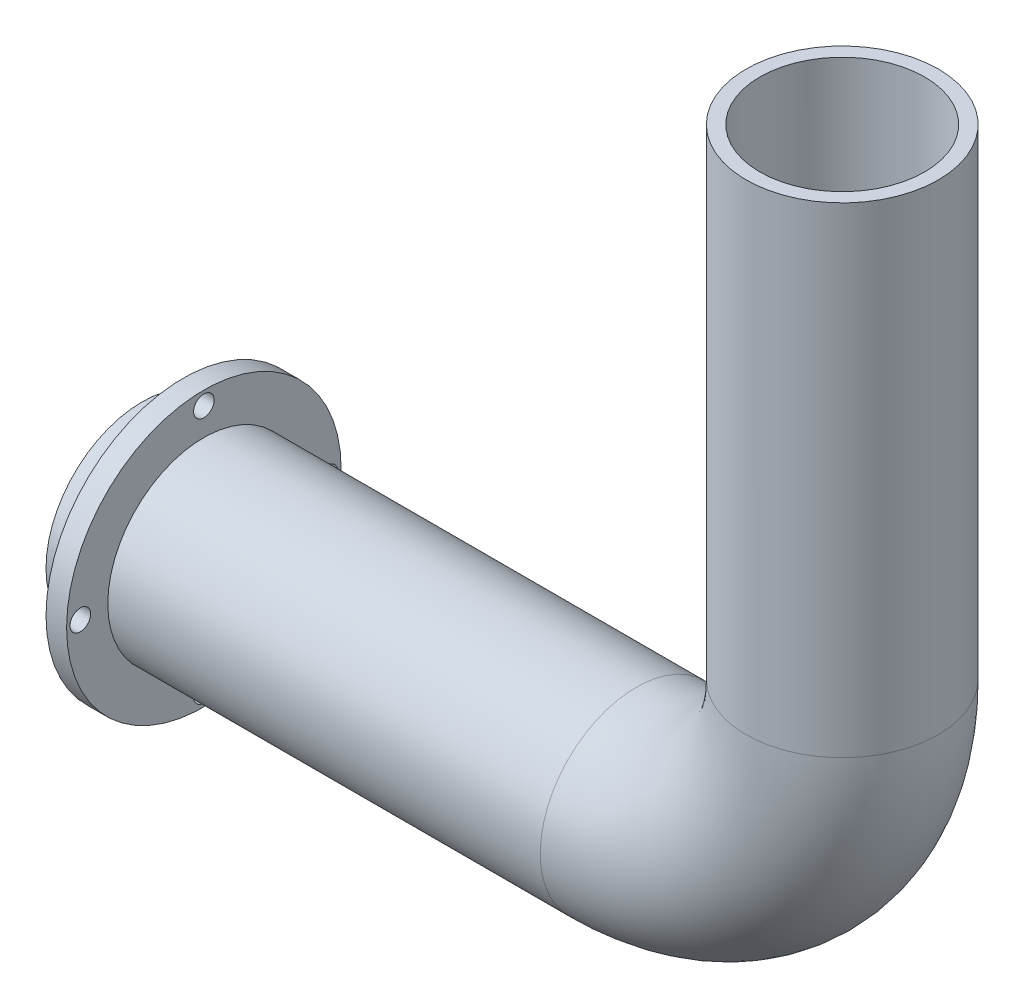
SolidWorks part; units mm, degrees
ref_plane "Front Plane" through (0, 0, 0) normal (0, 0, 1) x (1, 0, 0)
ref_plane "Top Plane" through (0, 0, 0) normal (0, 1, 0) x (1, 0, 0)
ref_plane "Right Plane" through (0, 0, 0) normal (1, 0, 0) x (0, 0, -1)
sketch "Sketch1" plane through (0, 0, 0) normal (0, 0, 1) x (1, 0, 0)
  line L0 (0, 0) -> (0, -70)
  line L1 (-30, -100) -> (-102, -100)
  arc A0 (0, -70) -> (-30, -100) centre (-30, -70) cw
  point P6 (0, -100)
  dimension "D3" = 30
  dimension "D1" = 100
  dimension "D2" = 102
sweep "Sweep1" add path "Sketch1" circular profile diameter 28 parameters "D3"=28
shell "Shell1" thickness 2
sketch "Sketch6" plane through (-102, 0, 0) normal (-1, 0, 0) x (0, 0, 1)
  circle A0 centre (0, -100) radius 12
  circle A1 centre (0, -100) radius 20
  circle A2 centre (0, -82) radius 1.5
  circle A3 centre (18, -100) radius 1.5
  circle A4 centre (0, -118) radius 1.5
  circle A5 centre (-18, -100) radius 1.5
  point P15 (0, -100)
  dimension "D1" = 40
  dimension "D2" = 3
  dimension "D3" = 18
  dimension "D4" = 4
extrude "Boss-Extrude1" add sketch "Sketch6" against normal blind 3 from offset 6
